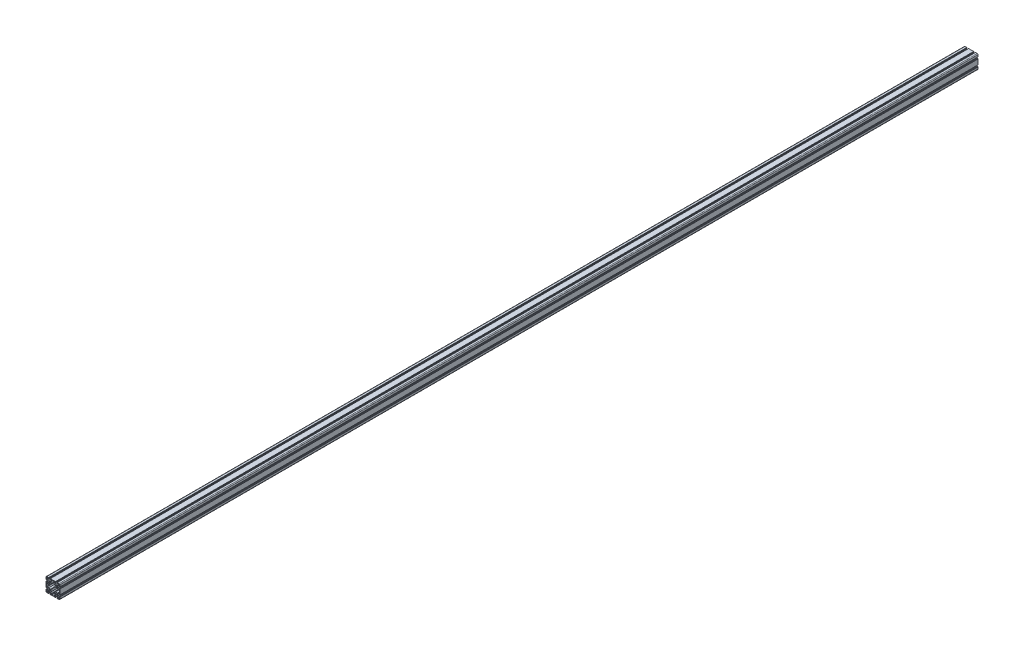
SolidWorks part; units mm, degrees
ref_plane "Front Plane" through (0, 0, 0) normal (0, 0, 1) x (1, 0, 0)
ref_plane "Top Plane" through (0, 0, 0) normal (0, 1, 0) x (1, 0, 0)
ref_plane "Right Plane" through (0, 0, 0) normal (1, 0, 0) x (0, 0, -1)
ref_plane "Plane1" through (0, 0, 100) normal (0, 0, 1) x (1, 0, 0)
sketch "Sketch1" plane through (0, 0, 100) normal (0, 0, 1) x (1, 0, 0)
  line L0 (-29.6117, 8.4562) -> (-25.1475, 12.9204)
  line L1 (-25.1475, 12.9204) -> (-14.0153, 12.9204)
  line L2 (-11.5153, 15.4204) -> (-11.5153, 26.5526)
  line L3 (-11.5153, 26.5526) -> (-7.0511, 31.0168)
  line L4 (-6.4653, 32.4311) -> (-6.4653, 37.4204)
  line L5 (-5.4653, 38.4204) -> (7.0347, 38.4204)
  line L6 (8.0347, 37.4204) -> (8.0347, 32.4311)
  line L7 (8.6205, 31.0168) -> (13.0847, 26.5526)
  line L8 (13.0847, 26.5526) -> (13.0847, 15.4204)
  line L9 (15.5847, 12.9204) -> (26.717, 12.9204)
  line L10 (26.717, 12.9204) -> (31.1812, 8.4562)
  line L11 (32.5954, 7.8704) -> (37.5847, 7.8704)
  line L12 (38.5847, 6.8704) -> (38.5847, -5.6296)
  line L13 (37.5847, -6.6296) -> (32.5954, -6.6296)
  line L14 (31.1812, -7.2154) -> (26.717, -11.6796)
  line L15 (26.717, -11.6796) -> (15.5847, -11.6796)
  line L16 (13.0847, -14.1796) -> (13.0847, -24.4834)
  line L17 (12.4989, -25.8976) -> (8.6205, -29.776)
  line L18 (8.0347, -31.1903) -> (8.0347, -36.1796)
  line L19 (7.0347, -37.1796) -> (-5.4653, -37.1796)
  line L20 (-6.4653, -36.1796) -> (-6.4653, -31.1903)
  line L21 (-7.0511, -29.776) -> (-11.5153, -25.3118)
  line L22 (-11.5153, -25.3118) -> (-11.5153, -14.1796)
  line L23 (-14.0153, -11.6796) -> (-25.1475, -11.6796)
  line L24 (-25.1475, -11.6796) -> (-29.6117, -7.2154)
  line L25 (-31.0259, -6.6296) -> (-36.0153, -6.6296)
  line L26 (-37.0153, -5.6296) -> (-37.0153, 6.8704)
  line L27 (-36.0153, 7.8704) -> (-31.0259, 7.8704)
  line L28 (-35.2193, 39.1244) -> (-31.9653, 39.1244)
  line L29 (-30.9653, 38.1244) -> (-30.9653, 33.3704)
  line L30 (-31.9653, 32.3704) -> (-36.7193, 32.3704)
  line L31 (-37.7193, 33.3704) -> (-37.7193, 36.6244)
  line L32 (36.7887, -37.8836) -> (33.5347, -37.8836)
  line L33 (32.5347, -36.8836) -> (32.5347, -32.1296)
  line L34 (33.5347, -31.1296) -> (38.2887, -31.1296)
  line L35 (39.2887, -32.1296) -> (39.2887, -35.3836)
  line L36 (37.7847, 10.3704) -> (32.8025, 10.3704)
  line L37 (32.8025, 10.3704) -> (28.4847, 14.6882)
  line L38 (28.4847, 14.6882) -> (28.4847, 26.5526)
  line L39 (28.4847, 26.5526) -> (32.8025, 30.8704)
  line L40 (32.8025, 30.8704) -> (37.7847, 30.8704)
  line L41 (38.7847, 29.8704) -> (38.7847, 28.2204)
  line L42 (37.7847, 27.2204) -> (36.2847, 27.2204)
  line L43 (36.2847, 27.2204) -> (36.2847, 25.0204)
  line L44 (36.5847, 24.7204) -> (39.7847, 24.7204)
  line L45 (39.7847, 24.7204) -> (39.7847, 25.5204)
  line L46 (39.9847, 25.7204) -> (40.7847, 25.7204)
  line L47 (40.7847, 25.7204) -> (40.7847, 36.1204)
  line L48 (36.2847, 40.6204) -> (25.8847, 40.6204)
  line L49 (25.8847, 40.6204) -> (25.8847, 39.8204)
  line L50 (25.6847, 39.6204) -> (24.8847, 39.6204)
  line L51 (24.8847, 39.6204) -> (24.8847, 36.4204)
  line L52 (25.1847, 36.1204) -> (27.3847, 36.1204)
  line L53 (27.3847, 36.1204) -> (27.3847, 37.6204)
  line L54 (28.3847, 38.6204) -> (30.0347, 38.6204)
  line L55 (31.0347, 37.6204) -> (31.0347, 32.6382)
  line L56 (31.0347, 32.6382) -> (26.717, 28.3204)
  line L57 (26.717, 28.3204) -> (14.8525, 28.3204)
  line L58 (14.8525, 28.3204) -> (10.5347, 32.6382)
  line L59 (10.5347, 32.6382) -> (10.5347, 37.6204)
  line L60 (11.5347, 38.6204) -> (13.1847, 38.6204)
  line L61 (14.1847, 37.6204) -> (14.1847, 36.1204)
  line L62 (14.1847, 36.1204) -> (16.3847, 36.1204)
  line L63 (16.6847, 36.4204) -> (16.6847, 39.6204)
  line L64 (16.6847, 39.6204) -> (15.8847, 39.6204)
  line L65 (15.6847, 39.8204) -> (15.6847, 40.6204)
  line L66 (15.6847, 40.6204) -> (-14.1153, 40.6204)
  line L67 (-14.1153, 40.6204) -> (-14.1153, 39.8204)
  line L68 (-14.3153, 39.6204) -> (-15.1153, 39.6204)
  line L69 (-15.1153, 39.6204) -> (-15.1153, 36.4204)
  line L70 (-14.8153, 36.1204) -> (-12.6153, 36.1204)
  line L71 (-12.6153, 36.1204) -> (-12.6153, 37.6204)
  line L72 (-11.6153, 38.6204) -> (-9.9653, 38.6204)
  line L73 (-8.9653, 37.6204) -> (-8.9653, 32.6382)
  line L74 (-8.9653, 32.6382) -> (-13.283, 28.3204)
  line L75 (-13.283, 28.3204) -> (-25.1475, 28.3204)
  line L76 (-25.1475, 28.3204) -> (-29.4653, 32.6382)
  line L77 (-29.4653, 32.6382) -> (-29.4653, 37.6204)
  line L78 (-28.4653, 38.6204) -> (-26.8153, 38.6204)
  line L79 (-25.8153, 37.6204) -> (-25.8153, 36.1204)
  line L80 (-25.8153, 36.1204) -> (-23.6153, 36.1204)
  line L81 (-23.3153, 36.4204) -> (-23.3153, 39.6204)
  line L82 (-23.3153, 39.6204) -> (-24.1153, 39.6204)
  line L83 (-24.3153, 39.8204) -> (-24.3153, 40.6204)
  line L84 (-24.3153, 40.6204) -> (-34.7153, 40.6204)
  line L85 (-39.2153, 36.1204) -> (-39.2153, 25.7204)
  line L86 (-39.2153, 25.7204) -> (-38.4153, 25.7204)
  line L87 (-38.2153, 25.5204) -> (-38.2153, 24.7204)
  line L88 (-38.2153, 24.7204) -> (-35.0153, 24.7204)
  line L89 (-34.7153, 25.0204) -> (-34.7153, 27.2204)
  line L90 (-34.7153, 27.2204) -> (-36.2153, 27.2204)
  line L91 (-37.2153, 28.2204) -> (-37.2153, 29.8704)
  line L92 (-36.2153, 30.8704) -> (-31.233, 30.8704)
  line L93 (-31.233, 30.8704) -> (-26.9153, 26.5526)
  line L94 (-26.9153, 26.5526) -> (-26.9153, 14.6882)
  line L95 (-26.9153, 14.6882) -> (-31.233, 10.3704)
  line L96 (-31.233, 10.3704) -> (-36.2153, 10.3704)
  line L97 (-37.2153, 11.3704) -> (-37.2153, 13.0204)
  line L98 (-36.2153, 14.0204) -> (-34.7153, 14.0204)
  line L99 (-34.7153, 14.0204) -> (-34.7153, 16.2204)
  line L100 (-35.0153, 16.5204) -> (-38.2153, 16.5204)
  line L101 (-38.2153, 16.5204) -> (-38.2153, 15.7204)
  line L102 (-38.4153, 15.5204) -> (-39.2153, 15.5204)
  line L103 (-39.2153, 15.5204) -> (-39.2153, -14.2796)
  line L104 (-39.2153, -14.2796) -> (-38.4153, -14.2796)
  line L105 (-38.2153, -14.4796) -> (-38.2153, -15.2796)
  line L106 (-38.2153, -15.2796) -> (-35.0153, -15.2796)
  line L107 (-34.7153, -14.9796) -> (-34.7153, -12.7796)
  line L108 (-34.7153, -12.7796) -> (-36.2153, -12.7796)
  line L109 (-37.2153, -11.7796) -> (-37.2153, -10.1296)
  line L110 (-36.2153, -9.1296) -> (-31.233, -9.1296)
  line L111 (-31.233, -9.1296) -> (-26.9153, -13.4474)
  line L112 (-26.9153, -13.4474) -> (-26.9153, -25.3118)
  line L113 (-26.9153, -25.3118) -> (-31.233, -29.6296)
  line L114 (-31.233, -29.6296) -> (-36.2153, -29.6296)
  line L115 (-37.2153, -28.6296) -> (-37.2153, -26.9796)
  line L116 (-36.2153, -25.9796) -> (-34.7153, -25.9796)
  line L117 (-34.7153, -25.9796) -> (-34.7153, -23.7796)
  line L118 (-35.0153, -23.4796) -> (-38.2153, -23.4796)
  line L119 (-38.2153, -23.4796) -> (-38.2153, -24.2796)
  line L120 (-38.4153, -24.4796) -> (-39.2153, -24.4796)
  line L121 (-39.2153, -24.4796) -> (-39.2153, -34.8796)
  line L122 (-34.7153, -39.3796) -> (-24.3153, -39.3796)
  line L123 (-24.3153, -39.3796) -> (-24.3153, -38.5796)
  line L124 (-24.1153, -38.3796) -> (-23.3153, -38.3796)
  line L125 (-23.3153, -38.3796) -> (-23.3153, -35.1796)
  line L126 (-23.6153, -34.8796) -> (-25.8153, -34.8796)
  line L127 (-25.8153, -34.8796) -> (-25.8153, -36.3796)
  line L128 (-26.8153, -37.3796) -> (-28.4653, -37.3796)
  line L129 (-29.4653, -36.3796) -> (-29.4653, -31.3974)
  line L130 (-29.4653, -31.3974) -> (-25.1475, -27.0796)
  line L131 (-25.1475, -27.0796) -> (-13.283, -27.0796)
  line L132 (-13.283, -27.0796) -> (-8.9653, -31.3974)
  line L133 (-8.9653, -31.3974) -> (-8.9653, -36.3796)
  line L134 (-9.9653, -37.3796) -> (-11.6153, -37.3796)
  line L135 (-12.6153, -36.3796) -> (-12.6153, -34.8796)
  line L136 (-12.6153, -34.8796) -> (-14.8153, -34.8796)
  line L137 (-15.1153, -35.1796) -> (-15.1153, -38.3796)
  line L138 (-15.1153, -38.3796) -> (-14.3153, -38.3796)
  line L139 (-14.1153, -38.5796) -> (-14.1153, -39.3796)
  line L140 (-14.1153, -39.3796) -> (15.6847, -39.3796)
  line L141 (15.6847, -39.3796) -> (15.6847, -38.5796)
  line L142 (15.8847, -38.3796) -> (16.6847, -38.3796)
  line L143 (16.6847, -38.3796) -> (16.6847, -35.1796)
  line L144 (16.3847, -34.8796) -> (14.1847, -34.8796)
  line L145 (14.1847, -34.8796) -> (14.1847, -36.3796)
  line L146 (13.1847, -37.3796) -> (11.5347, -37.3796)
  line L147 (10.5347, -36.3796) -> (10.5347, -31.3974)
  line L148 (10.5347, -31.3974) -> (14.8525, -27.0796)
  line L149 (14.8525, -27.0796) -> (26.717, -27.0796)
  line L150 (26.717, -27.0796) -> (31.0347, -31.3974)
  line L151 (31.0347, -31.3974) -> (31.0347, -36.3796)
  line L152 (30.0347, -37.3796) -> (28.3847, -37.3796)
  line L153 (27.3847, -36.3796) -> (27.3847, -34.8796)
  line L154 (27.3847, -34.8796) -> (25.1847, -34.8796)
  line L155 (24.8847, -35.1796) -> (24.8847, -38.3796)
  line L156 (24.8847, -38.3796) -> (25.6847, -38.3796)
  line L157 (25.8847, -38.5796) -> (25.8847, -39.3796)
  line L158 (25.8847, -39.3796) -> (36.2847, -39.3796)
  line L159 (40.7847, -34.8796) -> (40.7847, -24.4796)
  line L160 (40.7847, -24.4796) -> (39.9847, -24.4796)
  line L161 (39.7847, -24.2796) -> (39.7847, -23.4796)
  line L162 (39.7847, -23.4796) -> (36.5847, -23.4796)
  line L163 (36.2847, -23.7796) -> (36.2847, -25.9796)
  line L164 (36.2847, -25.9796) -> (37.7847, -25.9796)
  line L165 (38.7847, -26.9796) -> (38.7847, -28.6296)
  line L166 (37.7847, -29.6296) -> (32.8025, -29.6296)
  line L167 (32.8025, -29.6296) -> (28.4847, -25.3118)
  line L168 (28.4847, -25.3118) -> (28.4847, -13.4474)
  line L169 (28.4847, -13.4474) -> (32.8025, -9.1296)
  line L170 (32.8025, -9.1296) -> (37.7847, -9.1296)
  line L171 (38.7847, -10.1296) -> (38.7847, -11.7796)
  line L172 (37.7847, -12.7796) -> (36.2847, -12.7796)
  line L173 (36.2847, -12.7796) -> (36.2847, -14.9796)
  line L174 (36.5847, -15.2796) -> (39.7847, -15.2796)
  line L175 (39.7847, -15.2796) -> (39.7847, -14.4796)
  line L176 (39.9847, -14.2796) -> (40.7847, -14.2796)
  line L177 (40.7847, -14.2796) -> (40.7847, 15.5204)
  line L178 (40.7847, 15.5204) -> (39.9847, 15.5204)
  line L179 (39.7847, 15.7204) -> (39.7847, 16.5204)
  line L180 (39.7847, 16.5204) -> (36.5847, 16.5204)
  line L181 (36.2847, 16.2204) -> (36.2847, 14.0204)
  line L182 (36.2847, 14.0204) -> (37.7847, 14.0204)
  line L183 (38.7847, 13.0204) -> (38.7847, 11.3704)
  line L184 (-37.7193, -35.3836) -> (-37.7193, -32.1296)
  line L185 (-36.7193, -31.1296) -> (-31.9653, -31.1296)
  line L186 (-30.9653, -32.1296) -> (-30.9653, -36.8836)
  line L187 (-31.9653, -37.8836) -> (-35.2193, -37.8836)
  line L188 (39.2887, 36.6244) -> (39.2887, 33.3704)
  line L189 (38.2887, 32.3704) -> (33.5347, 32.3704)
  line L190 (32.5347, 33.3704) -> (32.5347, 38.1244)
  line L191 (33.5347, 39.1244) -> (36.7887, 39.1244)
  arc A0 (-14.0153, 12.9204) -> (-11.5153, 15.4204) centre (-14.0153, 15.4204) ccw
  arc A1 (-7.0511, 31.0168) -> (-6.4653, 32.4311) centre (-8.4653, 32.4311) ccw
  arc A2 (-6.4653, 37.4204) -> (-5.4653, 38.4204) centre (-5.4653, 37.4204) cw
  arc A3 (7.0347, 38.4204) -> (8.0347, 37.4204) centre (7.0347, 37.4204) cw
  arc A4 (8.0347, 32.4311) -> (8.6205, 31.0168) centre (10.0347, 32.4311) ccw
  arc A5 (13.0847, 15.4204) -> (15.5847, 12.9204) centre (15.5847, 15.4204) ccw
  arc A6 (31.1812, 8.4562) -> (32.5954, 7.8704) centre (32.5954, 9.8704) ccw
  arc A7 (37.5847, 7.8704) -> (38.5847, 6.8704) centre (37.5847, 6.8704) cw
  arc A8 (38.5847, -5.6296) -> (37.5847, -6.6296) centre (37.5847, -5.6296) cw
  arc A9 (32.5954, -6.6296) -> (31.1812, -7.2154) centre (32.5954, -8.6296) ccw
  arc A10 (15.5847, -11.6796) -> (13.0847, -14.1796) centre (15.5847, -14.1796) ccw
  arc A11 (13.0847, -24.4834) -> (12.4989, -25.8976) centre (11.0847, -24.4834) cw
  arc A12 (8.6205, -29.776) -> (8.0347, -31.1903) centre (10.0347, -31.1903) ccw
  arc A13 (8.0347, -36.1796) -> (7.0347, -37.1796) centre (7.0347, -36.1796) cw
  arc A14 (-5.4653, -37.1796) -> (-6.4653, -36.1796) centre (-5.4653, -36.1796) cw
  arc A15 (-6.4653, -31.1903) -> (-7.0511, -29.776) centre (-8.4653, -31.1903) ccw
  arc A16 (-11.5153, -14.1796) -> (-14.0153, -11.6796) centre (-14.0153, -14.1796) ccw
  arc A17 (-29.6117, -7.2154) -> (-31.0259, -6.6296) centre (-31.0259, -8.6296) ccw
  arc A18 (-36.0153, -6.6296) -> (-37.0153, -5.6296) centre (-36.0153, -5.6296) cw
  arc A19 (-37.0153, 6.8704) -> (-36.0153, 7.8704) centre (-36.0153, 6.8704) cw
  arc A20 (-31.0259, 7.8704) -> (-29.6117, 8.4562) centre (-31.0259, 9.8704) ccw
  arc A21 (-31.9653, 39.1244) -> (-30.9653, 38.1244) centre (-31.9653, 38.1244) cw
  arc A22 (-30.9653, 33.3704) -> (-31.9653, 32.3704) centre (-31.9653, 33.3704) cw
  arc A23 (-36.7193, 32.3704) -> (-37.7193, 33.3704) centre (-36.7193, 33.3704) cw
  arc A24 (-37.7193, 36.6244) -> (-35.2193, 39.1244) centre (-35.2193, 36.6244) cw
  circle A25 centre (-19.2153, -19.3796) radius 3.4
  circle A26 centre (20.7847, -19.3796) radius 3.4
  arc A27 (33.5347, -37.8836) -> (32.5347, -36.8836) centre (33.5347, -36.8836) cw
  arc A28 (32.5347, -32.1296) -> (33.5347, -31.1296) centre (33.5347, -32.1296) cw
  arc A29 (38.2887, -31.1296) -> (39.2887, -32.1296) centre (38.2887, -32.1296) cw
  arc A30 (39.2887, -35.3836) -> (36.7887, -37.8836) centre (36.7887, -35.3836) cw
  arc A31 (37.7847, 30.8704) -> (38.7847, 29.8704) centre (37.7847, 29.8704) cw
  arc A32 (38.7847, 28.2204) -> (37.7847, 27.2204) centre (37.7847, 28.2204) cw
  arc A33 (36.2847, 25.0204) -> (36.5847, 24.7204) centre (36.5847, 25.0204) ccw
  arc A34 (39.7847, 25.5204) -> (39.9847, 25.7204) centre (39.9847, 25.5204) cw
  arc A35 (40.7847, 36.1204) -> (36.2847, 40.6204) centre (36.2847, 36.1204) ccw
  arc A36 (25.8847, 39.8204) -> (25.6847, 39.6204) centre (25.6847, 39.8204) cw
  arc A37 (24.8847, 36.4204) -> (25.1847, 36.1204) centre (25.1847, 36.4204) ccw
  arc A38 (27.3847, 37.6204) -> (28.3847, 38.6204) centre (28.3847, 37.6204) cw
  arc A39 (30.0347, 38.6204) -> (31.0347, 37.6204) centre (30.0347, 37.6204) cw
  arc A40 (10.5347, 37.6204) -> (11.5347, 38.6204) centre (11.5347, 37.6204) cw
  arc A41 (13.1847, 38.6204) -> (14.1847, 37.6204) centre (13.1847, 37.6204) cw
  arc A42 (16.3847, 36.1204) -> (16.6847, 36.4204) centre (16.3847, 36.4204) ccw
  arc A43 (15.8847, 39.6204) -> (15.6847, 39.8204) centre (15.8847, 39.8204) cw
  arc A44 (-14.1153, 39.8204) -> (-14.3153, 39.6204) centre (-14.3153, 39.8204) cw
  arc A45 (-15.1153, 36.4204) -> (-14.8153, 36.1204) centre (-14.8153, 36.4204) ccw
  arc A46 (-12.6153, 37.6204) -> (-11.6153, 38.6204) centre (-11.6153, 37.6204) cw
  arc A47 (-9.9653, 38.6204) -> (-8.9653, 37.6204) centre (-9.9653, 37.6204) cw
  arc A48 (-29.4653, 37.6204) -> (-28.4653, 38.6204) centre (-28.4653, 37.6204) cw
  arc A49 (-26.8153, 38.6204) -> (-25.8153, 37.6204) centre (-26.8153, 37.6204) cw
  arc A50 (-23.6153, 36.1204) -> (-23.3153, 36.4204) centre (-23.6153, 36.4204) ccw
  arc A51 (-24.1153, 39.6204) -> (-24.3153, 39.8204) centre (-24.1153, 39.8204) cw
  arc A52 (-34.7153, 40.6204) -> (-39.2153, 36.1204) centre (-34.7153, 36.1204) ccw
  arc A53 (-38.4153, 25.7204) -> (-38.2153, 25.5204) centre (-38.4153, 25.5204) cw
  arc A54 (-35.0153, 24.7204) -> (-34.7153, 25.0204) centre (-35.0153, 25.0204) ccw
  arc A55 (-36.2153, 27.2204) -> (-37.2153, 28.2204) centre (-36.2153, 28.2204) cw
  arc A56 (-37.2153, 29.8704) -> (-36.2153, 30.8704) centre (-36.2153, 29.8704) cw
  arc A57 (-36.2153, 10.3704) -> (-37.2153, 11.3704) centre (-36.2153, 11.3704) cw
  arc A58 (-37.2153, 13.0204) -> (-36.2153, 14.0204) centre (-36.2153, 13.0204) cw
  arc A59 (-34.7153, 16.2204) -> (-35.0153, 16.5204) centre (-35.0153, 16.2204) ccw
  arc A60 (-38.2153, 15.7204) -> (-38.4153, 15.5204) centre (-38.4153, 15.7204) cw
  arc A61 (-38.4153, -14.2796) -> (-38.2153, -14.4796) centre (-38.4153, -14.4796) cw
  arc A62 (-35.0153, -15.2796) -> (-34.7153, -14.9796) centre (-35.0153, -14.9796) ccw
  arc A63 (-36.2153, -12.7796) -> (-37.2153, -11.7796) centre (-36.2153, -11.7796) cw
  arc A64 (-37.2153, -10.1296) -> (-36.2153, -9.1296) centre (-36.2153, -10.1296) cw
  arc A65 (-36.2153, -29.6296) -> (-37.2153, -28.6296) centre (-36.2153, -28.6296) cw
  arc A66 (-37.2153, -26.9796) -> (-36.2153, -25.9796) centre (-36.2153, -26.9796) cw
  arc A67 (-34.7153, -23.7796) -> (-35.0153, -23.4796) centre (-35.0153, -23.7796) ccw
  arc A68 (-38.2153, -24.2796) -> (-38.4153, -24.4796) centre (-38.4153, -24.2796) cw
  arc A69 (-39.2153, -34.8796) -> (-34.7153, -39.3796) centre (-34.7153, -34.8796) ccw
  arc A70 (-24.3153, -38.5796) -> (-24.1153, -38.3796) centre (-24.1153, -38.5796) cw
  arc A71 (-23.3153, -35.1796) -> (-23.6153, -34.8796) centre (-23.6153, -35.1796) ccw
  arc A72 (-25.8153, -36.3796) -> (-26.8153, -37.3796) centre (-26.8153, -36.3796) cw
  arc A73 (-28.4653, -37.3796) -> (-29.4653, -36.3796) centre (-28.4653, -36.3796) cw
  arc A74 (-8.9653, -36.3796) -> (-9.9653, -37.3796) centre (-9.9653, -36.3796) cw
  arc A75 (-11.6153, -37.3796) -> (-12.6153, -36.3796) centre (-11.6153, -36.3796) cw
  arc A76 (-14.8153, -34.8796) -> (-15.1153, -35.1796) centre (-14.8153, -35.1796) ccw
  arc A77 (-14.3153, -38.3796) -> (-14.1153, -38.5796) centre (-14.3153, -38.5796) cw
  arc A78 (15.6847, -38.5796) -> (15.8847, -38.3796) centre (15.8847, -38.5796) cw
  arc A79 (16.6847, -35.1796) -> (16.3847, -34.8796) centre (16.3847, -35.1796) ccw
  arc A80 (14.1847, -36.3796) -> (13.1847, -37.3796) centre (13.1847, -36.3796) cw
  arc A81 (11.5347, -37.3796) -> (10.5347, -36.3796) centre (11.5347, -36.3796) cw
  arc A82 (31.0347, -36.3796) -> (30.0347, -37.3796) centre (30.0347, -36.3796) cw
  arc A83 (28.3847, -37.3796) -> (27.3847, -36.3796) centre (28.3847, -36.3796) cw
  arc A84 (25.1847, -34.8796) -> (24.8847, -35.1796) centre (25.1847, -35.1796) ccw
  arc A85 (25.6847, -38.3796) -> (25.8847, -38.5796) centre (25.6847, -38.5796) cw
  arc A86 (36.2847, -39.3796) -> (40.7847, -34.8796) centre (36.2847, -34.8796) ccw
  arc A87 (39.9847, -24.4796) -> (39.7847, -24.2796) centre (39.9847, -24.2796) cw
  arc A88 (36.5847, -23.4796) -> (36.2847, -23.7796) centre (36.5847, -23.7796) ccw
  arc A89 (37.7847, -25.9796) -> (38.7847, -26.9796) centre (37.7847, -26.9796) cw
  arc A90 (38.7847, -28.6296) -> (37.7847, -29.6296) centre (37.7847, -28.6296) cw
  arc A91 (37.7847, -9.1296) -> (38.7847, -10.1296) centre (37.7847, -10.1296) cw
  arc A92 (38.7847, -11.7796) -> (37.7847, -12.7796) centre (37.7847, -11.7796) cw
  arc A93 (36.2847, -14.9796) -> (36.5847, -15.2796) centre (36.5847, -14.9796) ccw
  arc A94 (39.7847, -14.4796) -> (39.9847, -14.2796) centre (39.9847, -14.4796) cw
  arc A95 (39.9847, 15.5204) -> (39.7847, 15.7204) centre (39.9847, 15.7204) cw
  arc A96 (36.5847, 16.5204) -> (36.2847, 16.2204) centre (36.5847, 16.2204) ccw
  arc A97 (37.7847, 14.0204) -> (38.7847, 13.0204) centre (37.7847, 13.0204) cw
  arc A98 (38.7847, 11.3704) -> (37.7847, 10.3704) centre (37.7847, 11.3704) cw
  arc A99 (-37.7193, -32.1296) -> (-36.7193, -31.1296) centre (-36.7193, -32.1296) cw
  arc A100 (-31.9653, -31.1296) -> (-30.9653, -32.1296) centre (-31.9653, -32.1296) cw
  arc A101 (-30.9653, -36.8836) -> (-31.9653, -37.8836) centre (-31.9653, -36.8836) cw
  arc A102 (-35.2193, -37.8836) -> (-37.7193, -35.3836) centre (-35.2193, -35.3836) cw
  arc A103 (39.2887, 33.3704) -> (38.2887, 32.3704) centre (38.2887, 33.3704) cw
  arc A104 (33.5347, 32.3704) -> (32.5347, 33.3704) centre (33.5347, 33.3704) cw
  arc A105 (32.5347, 38.1244) -> (33.5347, 39.1244) centre (33.5347, 38.1244) cw
  arc A106 (36.7887, 39.1244) -> (39.2887, 36.6244) centre (36.7887, 36.6244) cw
  circle A107 centre (20.7847, 20.6204) radius 3.4
  circle A108 centre (-19.2153, 20.6204) radius 3.4
extrude "Boss-Extrude1" add sketch "Sketch1" against normal blind 5338
